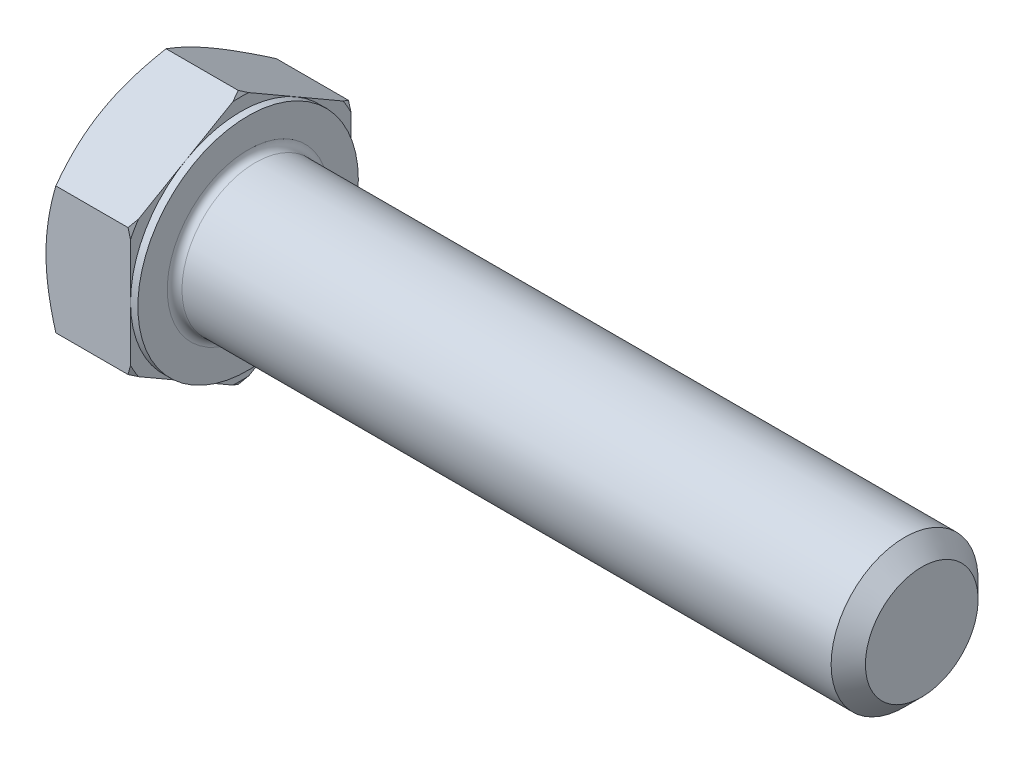
SolidWorks part; units mm, degrees
extrude "Base-Extrude" add sketch "Sketch1" along normal blind 7.5
sketch "Sketch1" plane through (0, 0, 0) normal (1, 0, 0) x (0, 0, -1)
  line L0 (9, 5.1962) -> (9, -5.1962)
  line L1 (-9, 5.1962) -> (-9, -5.1962)
  line L2 (9, -5.1962) -> (0, -10.3923)
  line L3 (0, -10.3923) -> (-9, -5.1962)
  line L4 (9, 5.1962) -> (0, 10.3923)
  line L5 (0, 10.3923) -> (-9, 5.1962)
revolve "Cut-Revolve1" cut sketch "Sketch3" angle 360 about L6
sketch "Sketch3" plane through (0, 0, 0) normal (0, 0, 1) x (1, 0, 0)
  line L0 (0, 9) -> (3.6906, 15.3923)
  line L1 (0, 10.3923) -> (0, 5.1962) construction
  line L2 (3.6906, 15.3923) -> (3.6906, 20.3923)
  line L3 (3.6906, 20.3923) -> (-10, 20.3923)
  line L4 (-10, 20.3923) -> (-10, 9)
  line L5 (-10, 9) -> (0, 9)
  line L6 (0, 0) -> (99.06, 0) construction
  line L7 (7.5, 10.3923) -> (0, 10.3923) construction
ref_plane "Front" through (0, 0, 0) normal (0, 0, 1) x (1, 0, 0)
ref_plane "Top" through (0, 0, 0) normal (0, 1, 0) x (1, 0, 0)
ref_plane "Right" through (0, 0, 0) normal (1, 0, 0) x (0, 0, -1)
sketch "Sketch2" plane through (0, 0, 0) normal (0, 0, 1) x (1, 0, 0)
  line L0 (0, 5.1962) -> (0, -5.1962) construction
  line L1 (0, 0) -> (62.5, 0)
  line L2 (0, 0) -> (0, 6)
  line L3 (0, 6) -> (7.7917, 6)
  line L4 (62.5, 0) -> (62.5, 4.4845)
  line L5 (7.5, 10.3923) -> (7.5, 5.1962) construction
  line L7 (0, 0) -> (96.52, 0) construction
  line L8 (62.5, -4.4845) -> (7.7917, -6) construction
  line L9 (0, -6) -> (7.7917, -6) construction
  line L10 (9.25, 15.24) -> (9.25, -1.27) construction
  line L11 (32.5, 15.24) -> (32.5, -1.27) construction
  line L12 (7.5, 5.1962) -> (7.5, -5.1962) construction
  line L13 (7.7917, 6) -> (62.5, 6)
  line L14 (62.5, 6) -> (62.5, 4.4845)
revolve "Boss-Revolve1" add sketch "Sketch2" angle 360 about L7
cosmetic thread "Helix1" parameters "Thread_length"=30, "Thread_minor"=8.969
sketch "Sketch5" plane through (0, 0, 0) normal (0, 0, 1) x (1, 0, 0)
  line L0 (7.5, 9) -> (3.8094, 15.3923)
  line L1 (7.5, 10.3923) -> (7.5, 5.1962) construction
  line L2 (3.8094, 15.3923) -> (3.8094, 20.3923)
  line L3 (3.8094, 20.3923) -> (13.8094, 20.3923)
  line L4 (13.8094, 20.3923) -> (13.8094, 9)
  line L5 (13.8094, 9) -> (7.5, 9)
  line L7 (7.5, 10.3923) -> (0.8038, 10.3923) construction
  line L8 (0, 0) -> (99.06, 0) construction
  line L9 (0, 0) -> (99.06, 0) construction
revolve "Cut-Revolve2" cut sketch "Sketch5" angle 360 about L8
sketch "Sketch4" plane through (0, 0, 0) normal (0, 0, 1) x (1, 0, 0)
  line L1 (7.5, 10.3923) -> (7.5, 5.1962) construction
  line L2 (7.5, 9) -> (6.9, 9)
  line L3 (7.5, 9) -> (7.5, 20.3923)
  line L4 (7.5, 20.3923) -> (6.9, 20.3923)
  line L5 (0, 0) -> (95.25, 0) construction
  line L6 (0, 0) -> (96.52, 0) construction
  line L7 (6.9, 9) -> (6.9, 20.3923)
  line L8 (6.6962, 10.3923) -> (0.8038, 10.3923) construction
revolve "Cut-Revolve3" cut sketch "Sketch4" angle 360 about L5
chamfer "Chamfer" distance 1.4 angle 45 1 edges at (62.5, 0, 6)
fillet "Fillet" radius 0.6 1 edges at (7.5, 0, -6)
sketch "Sketch6" plane through (0, 0, 0) normal (0, 0, 1) x (1, 0, 0)
  line L0 (32.5, -4.4845) -> (31.625, -6)
  line L1 (32.5, -4.4845) -> (33.375, -6)
  line L2 (33.375, -6) -> (33.375, -7.5)
  line L3 (-3.175, 0) -> (5.1513, 0) construction
  line L5 (33.375, -7.5) -> (31.625, -7.5)
  line L6 (31.625, -7.5) -> (31.625, -6)
revolve "Cut-Revolve4" [suppressed] cut sketch "Sketch6" angle 360 about L3
pattern_linear "LPattern1" [suppressed]
equation "\"D3@Sketch1\" = \"s@Sketch1\" / 2"
equation "\"D4@Sketch1\" = \"D3@Sketch1\""
equation "\"D5@Sketch1\" = \"D4@Sketch1\""
equation "\"Thread_minor@Helix1\" = \"Minor_dia@Sketch2\""
equation "\"D1@Sketch3\" = \"s@Sketch1\" / 2"
equation "\"D1@Sketch5\" = \"s@Sketch1\" / 2"
equation "\"Head_ch_ang@Sketch5\" = \"Head_ch_ang@Sketch3\""
equation "\"D1@Sketch4\" = \"s@Sketch1\""
equation "\"Thread_length@Helix1\" = ((sgn( (\"l@Sketch2\" - \"p@Sketch2\" ) - \"h@Sketch2\" )-1)*( (\"l@Sketch2\" - \"p@Sketch2\" ) - \"h@Sketch2\" ))/-2+ \"h@Sketch2\""
equation "\"Thread_minor@Sketch6\" = \"Minor_dia@Sketch2\""
equation "\"Diameter@Sketch6\" = \"m@Sketch2\""
equation "\"Overcut@Sketch6\" = \"m@Sketch2\" * 1.25"
equation "\"Start@Sketch6\" = \"k@Base-Extrude\" + \"l@Sketch2\" - \"Thread_length@Helix1\"  '---Non-countersunk---"
equation "\"Num_threads@LPattern1\" = int( \"Thread_length@Helix1\" / \"p@Sketch2\" + 0.999 )  + 1"
equation "\"Advance@LPattern1\" = \"Thread_length@Helix1\" /  (\"Num_threads@LPattern1\" - 1) 'relax it"
equation "\"Num_threads@LPattern1\" = \"Num_threads@LPattern1\" - sgn( \"Num_threads@LPattern1\" - 1) '---chamfered tips oxxx---"
equation "\"Minor_dia@Sketch2\" = \"m@Sketch2\"-\"p@Sketch2\" * 1.732"
equation "\"D1@Chamfer\" = \"p@Sketch2\"*0.8"
